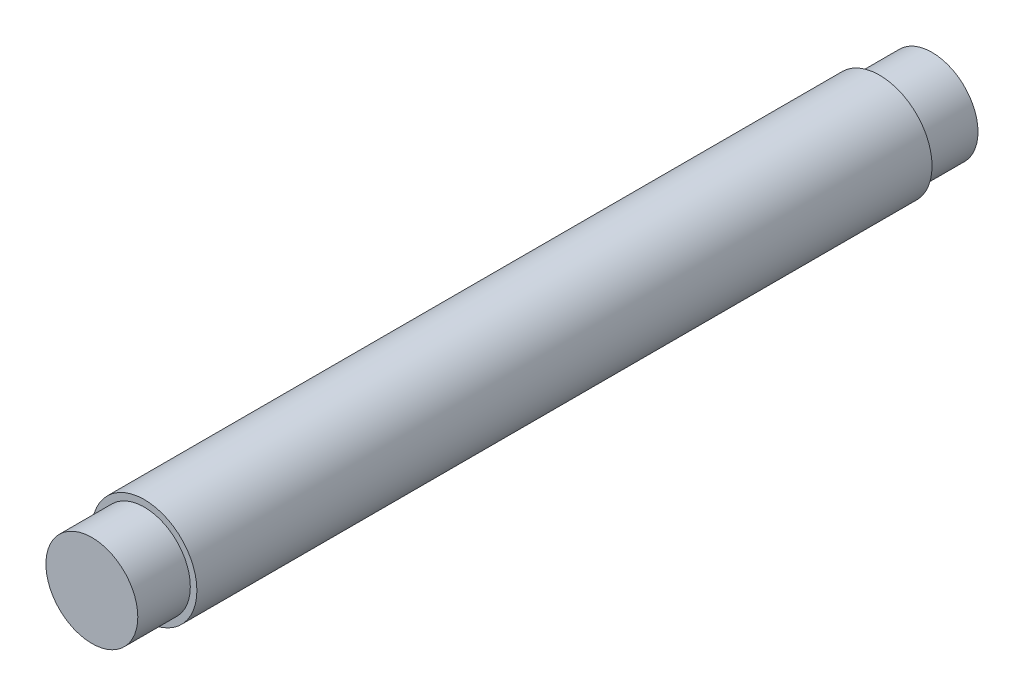
from build123d import *

# Parameters (mm, degrees)
SKETCH1_R           = 87.5
BOSS_EXTRUDE1_DEPTH = 800
SKETCH2_R           = 100
BOSS_EXTRUDE2_DEPTH = 700


with BuildPart() as part:
    # Sketch1 → Boss-Extrude1 (new, symmetric)
    with BuildSketch(Plane.XY):
        Circle(SKETCH1_R)
    extrude(amount=BOSS_EXTRUDE1_DEPTH, both=True)

    # Sketch2 → Boss-Extrude2 (add, symmetric)
    with BuildSketch(Plane.XY):
        Circle(SKETCH2_R)
    extrude(amount=BOSS_EXTRUDE2_DEPTH, both=True)


solid = part.part
